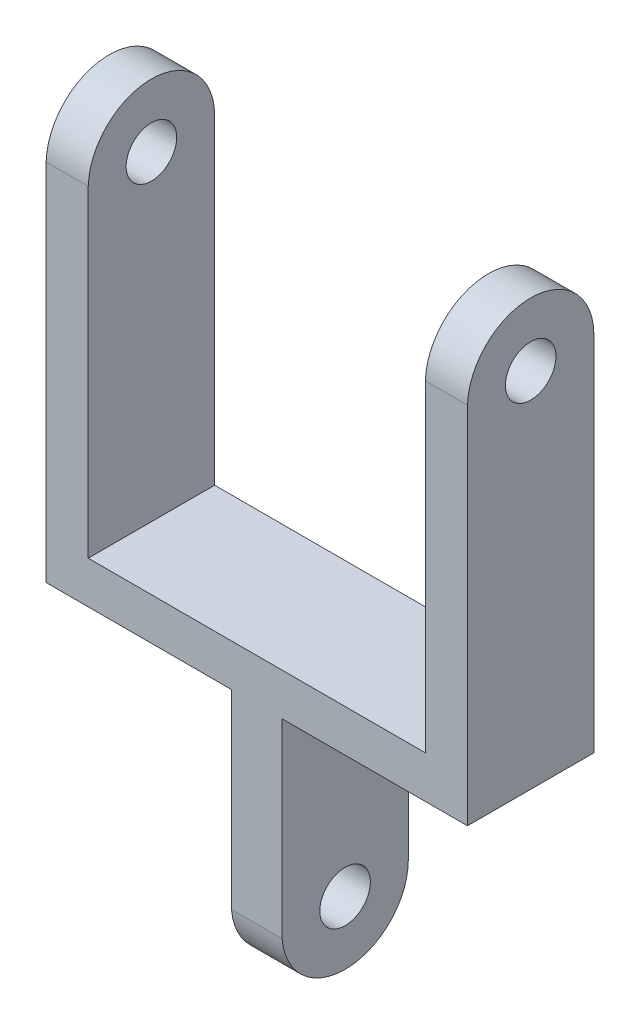
from build123d import *

# Parameters (mm, degrees)
BOSS_EXTRUDE1_DEPTH = 15
SKETCH2_R           = 3
CUT_EXTRUDE1_DEPTH  = 100.749686716


with BuildPart() as part:
    # Sketch1 → Boss-Extrude1 (new body)
    with BuildSketch(Plane.XY):
        Polygon((20, 35), (-20, 35), (-20, 85), (-25, 85), (-25, 30), (-3, 30), (-3, 0), (0, 0), (3, 0), (3, 30), (25, 30), (25, 85), (20, 85), align=None)
    extrude(amount=BOSS_EXTRUDE1_DEPTH)

    # Sketch2 → Cut-Extrude1 (cut, through all)
    with BuildSketch(Plane.ZY.offset(25)):
        with Locations(Location((7.503230167, 72.999996799, 0), (0, 0, 270))):
            Circle(SKETCH2_R)
        with Locations(Location((7.523630467, 8, 0), (0, 0, 270))):
            Circle(SKETCH2_R)
        with BuildLine():
            Line((0.003230167, 72.999996799), (-23.0886588, 76.719933094))
            Line((-23.0886588, 76.719933094), (-0.661840838, 109.961720022))
            Line((-0.661840838, 109.961720022), (34.957913296, 90.556615978))
            Line((34.957913296, 90.556615978), (15.003230167, 72.999996799))
            ThreePointArc((15.003230167, 72.999996799), (7.503230167, 80.499996799), (0.003230167, 72.999996799))
        make_face()
        with BuildLine():
            Line((0.023630467, 8), (-15.301630232, 0.607134927))
            Line((-15.301630232, 0.607134927), (-3.280552195, -15.592363972))
            Line((-3.280552195, -15.592363972), (32.469088575, -12.351899457))
            Line((32.469088575, -12.351899457), (24.841547467, 4.357134927))
            Line((24.841547467, 4.357134927), (15.023630467, 8))
            ThreePointArc((15.023630467, 8), (7.523630467, 0.5), (0.023630467, 8))
        make_face()
    extrude(amount=-CUT_EXTRUDE1_DEPTH, mode=Mode.SUBTRACT)


solid = part.part
